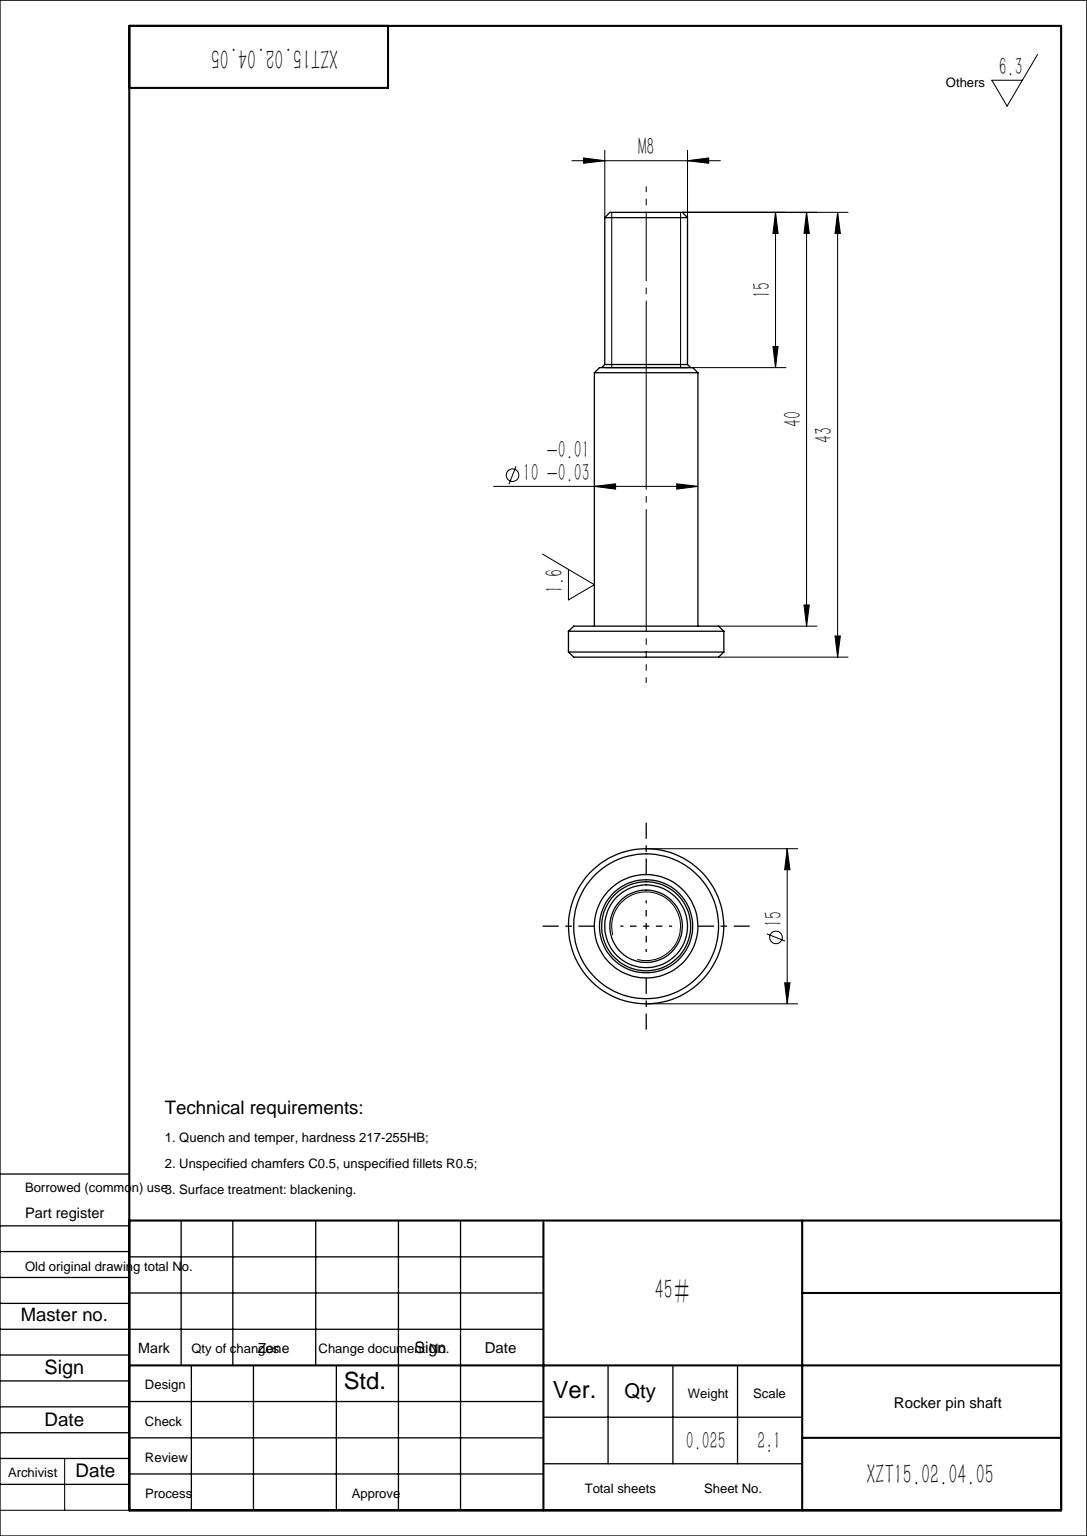
from build123d import *

# Parameters (mm, degrees)
CHAMFER1_SIZE = 0.5
CHAMFER2_SIZE = 0.3


with BuildPart() as part:
    # Sketch1 → Revolve1 (revolve)
    with BuildSketch(Plane.XY, mode=Mode.PRIVATE) as revolve1_sk:
        Polygon((0, 0), (7.5, 0), (7.5, 3), (5, 3), (5, 28), (4, 28), (4, 43), (0, 43), align=None)
    revolve(revolve1_sk.sketch.rotate(Axis((0, 0, 0), (0, -1, 0)), 90), axis=Axis((0, 0, 0), (0, -1, 0)))

    # Chamfer1
    chamfer1_edges = [part.edges().sort_by_distance(p)[0] for p in [
        (0, 43, -4),
        (0, 28, -5),
        (0, 3, -7.5),
        (0, 0, -7.5),
    ]]
    chamfer(chamfer1_edges, length=CHAMFER1_SIZE)

    # Chamfer2
    chamfer2_edges = [part.edges().sort_by_distance(p)[0] for p in [
        (0, 28, -4),
    ]]
    chamfer(chamfer2_edges, length=CHAMFER2_SIZE)


solid = part.part
